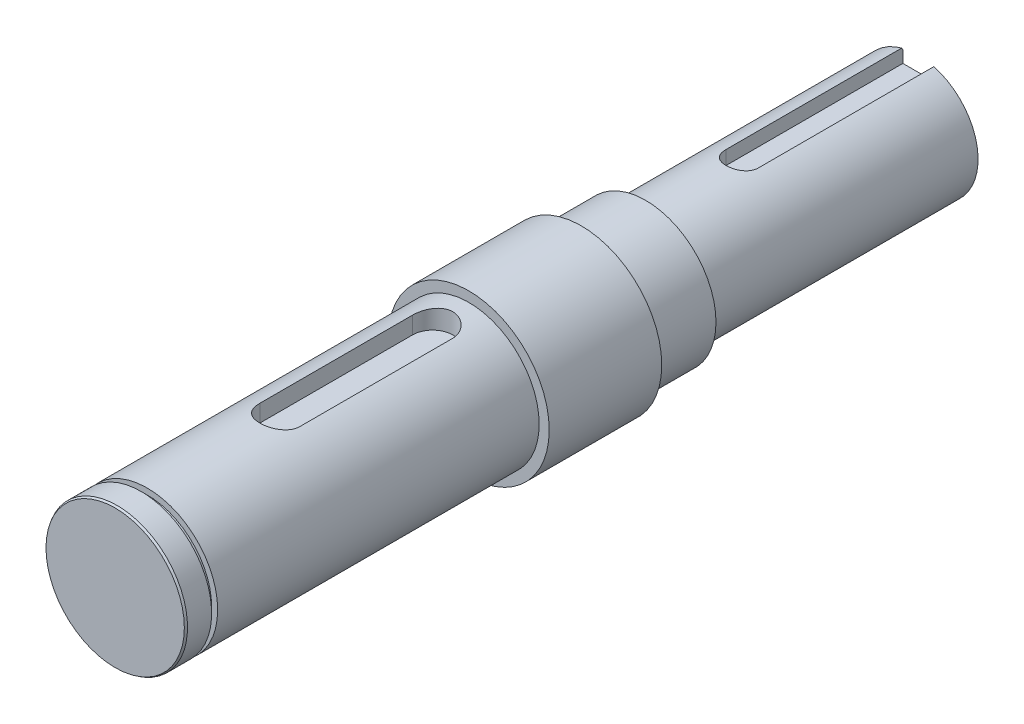
SolidWorks part; units mm, degrees
ref_plane "Front Plane" through (0, 0, 0) normal (0, 0, 1) x (1, 0, 0)
ref_plane "Top Plane" through (0, 0, 0) normal (0, 1, 0) x (1, 0, 0)
ref_plane "Right Plane" through (0, 0, 0) normal (1, 0, 0) x (0, 0, -1)
other "Configuration Table"
sketch "Sketch1" plane through (0, 0, 0) normal (0, 0, 1) x (1, 0, 0)
  circle A0 centre (0, 0) radius 15
  dimension "D1" = 30
extrude "Boss-Extrude1" add sketch "Sketch1" along normal blind 68
sketch "Sketch2" plane through (0, 0, 68) normal (0, 0, 1) x (1, 0, 0)
  circle A0 centre (0, 0) radius 17.5
  dimension "D1" = 35
extrude "Boss-Extrude2" add sketch "Sketch2" along normal blind 16
sketch "Sketch3" plane through (0, 0, 84) normal (0, 0, 1) x (1, 0, 0)
  circle A0 centre (0, 0) radius 20
  dimension "D1" = 40
extrude "Boss-Extrude3" add sketch "Sketch3" along normal blind 28
sketch "Sketch4" plane through (0, 0, 112) normal (0, 0, 1) x (1, 0, 0)
  circle A0 centre (0, 0) radius 17.5
  dimension "D1" = 35
extrude "Boss-Extrude4" add sketch "Sketch4" along normal blind 80
sketch "Sketch5" plane through (0, 0, 192) normal (0, 0, 1) x (1, 0, 0)
  circle A0 centre (0, 0) radius 16
  dimension "D1" = 32
extrude "Boss-Extrude5" add sketch "Sketch5" along normal blind 1.5
sketch "Sketch6" plane through (0, 0, 193.5) normal (0, 0, 1) x (1, 0, 0)
  circle A0 centre (0, 0) radius 17.5
  dimension "D1" = 35
extrude "Boss-Extrude6" add sketch "Sketch6" along normal blind 6.5
sketch "Sketch7" plane through (0, 0, 0) normal (0, 1, 0) x (1, 0, 0)
  line L0 (0, -159) -> (0, -121) construction
  line L1 (-5, -159) -> (-5, -121)
  line L2 (5, -159) -> (5, -121)
  line L3 (-17.5, -112) -> (17.5, -112) construction
  arc A0 (-5, -159) -> (5, -159) centre (0, -159) ccw
  arc A1 (5, -121) -> (-5, -121) centre (0, -121) ccw
  point P3 (0, -140)
  dimension "D3" = 5
  dimension "D1" = 38
  dimension "D2" = 9
extrude "Cut-Extrude1" cut sketch "Sketch7" against normal blind 5 from offset 17.5
sketch "Sketch8" plane through (0, 0, 0) normal (0, 1, 0) x (1, 0, 0)
  line L0 (0, -44) -> (0, 0) construction
  line L1 (-4, -44) -> (-4, 0)
  line L2 (4, -44) -> (4, 0)
  arc A0 (-4, -44) -> (4, -44) centre (0, -44) ccw
  arc A1 (4, 0) -> (-4, 0) centre (0, 0) ccw
  point P3 (0, -22)
  dimension "D2" = 4
  dimension "D1" = 44
extrude "Cut-Extrude2" cut sketch "Sketch8" against normal blind 4 from offset 15
sketch "Sketch9" plane through (0, 0, 0) normal (0, 1, 0) x (1, 0, 0)
  line L0 (0, -61) -> (0, -54) construction
  line L1 (-4, -61) -> (-4, -54)
  line L2 (4, -61) -> (4, -54)
  line L3 (17.5, -68) -> (-17.5, -68) construction
  arc A0 (-4, -61) -> (4, -61) centre (0, -61) ccw
  arc A1 (4, -54) -> (-4, -54) centre (0, -54) ccw
  point P3 (0, -57.5)
  dimension "D2" = 4
  dimension "D1" = 7
  dimension "D3" = 7
extrude "Cut-Extrude3" cut sketch "Sketch9" along normal blind 4 from offset 15 offset against normal yes
chamfer "Chamfer1" distance 0.5 angle 30 2 edges at (17.5, 0, 200) (0, -15, 0)
